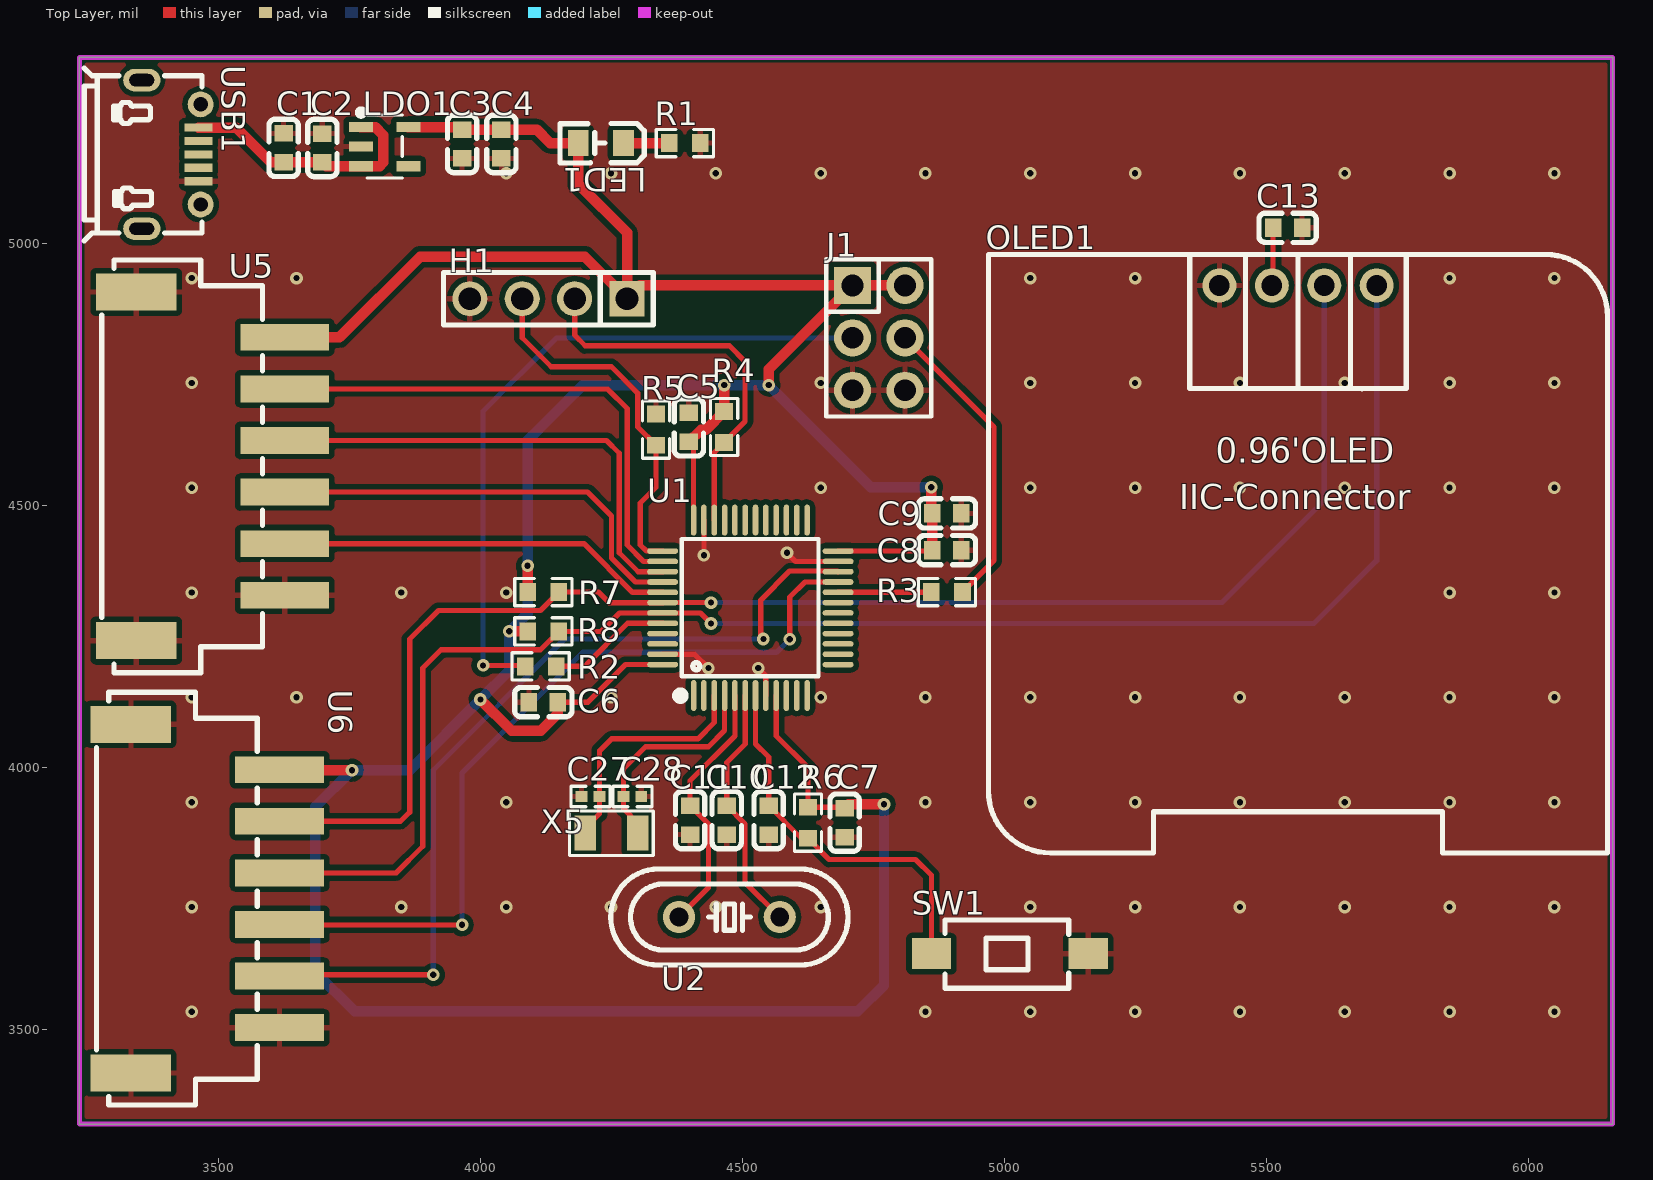
[diagram p0: Top Layer view]
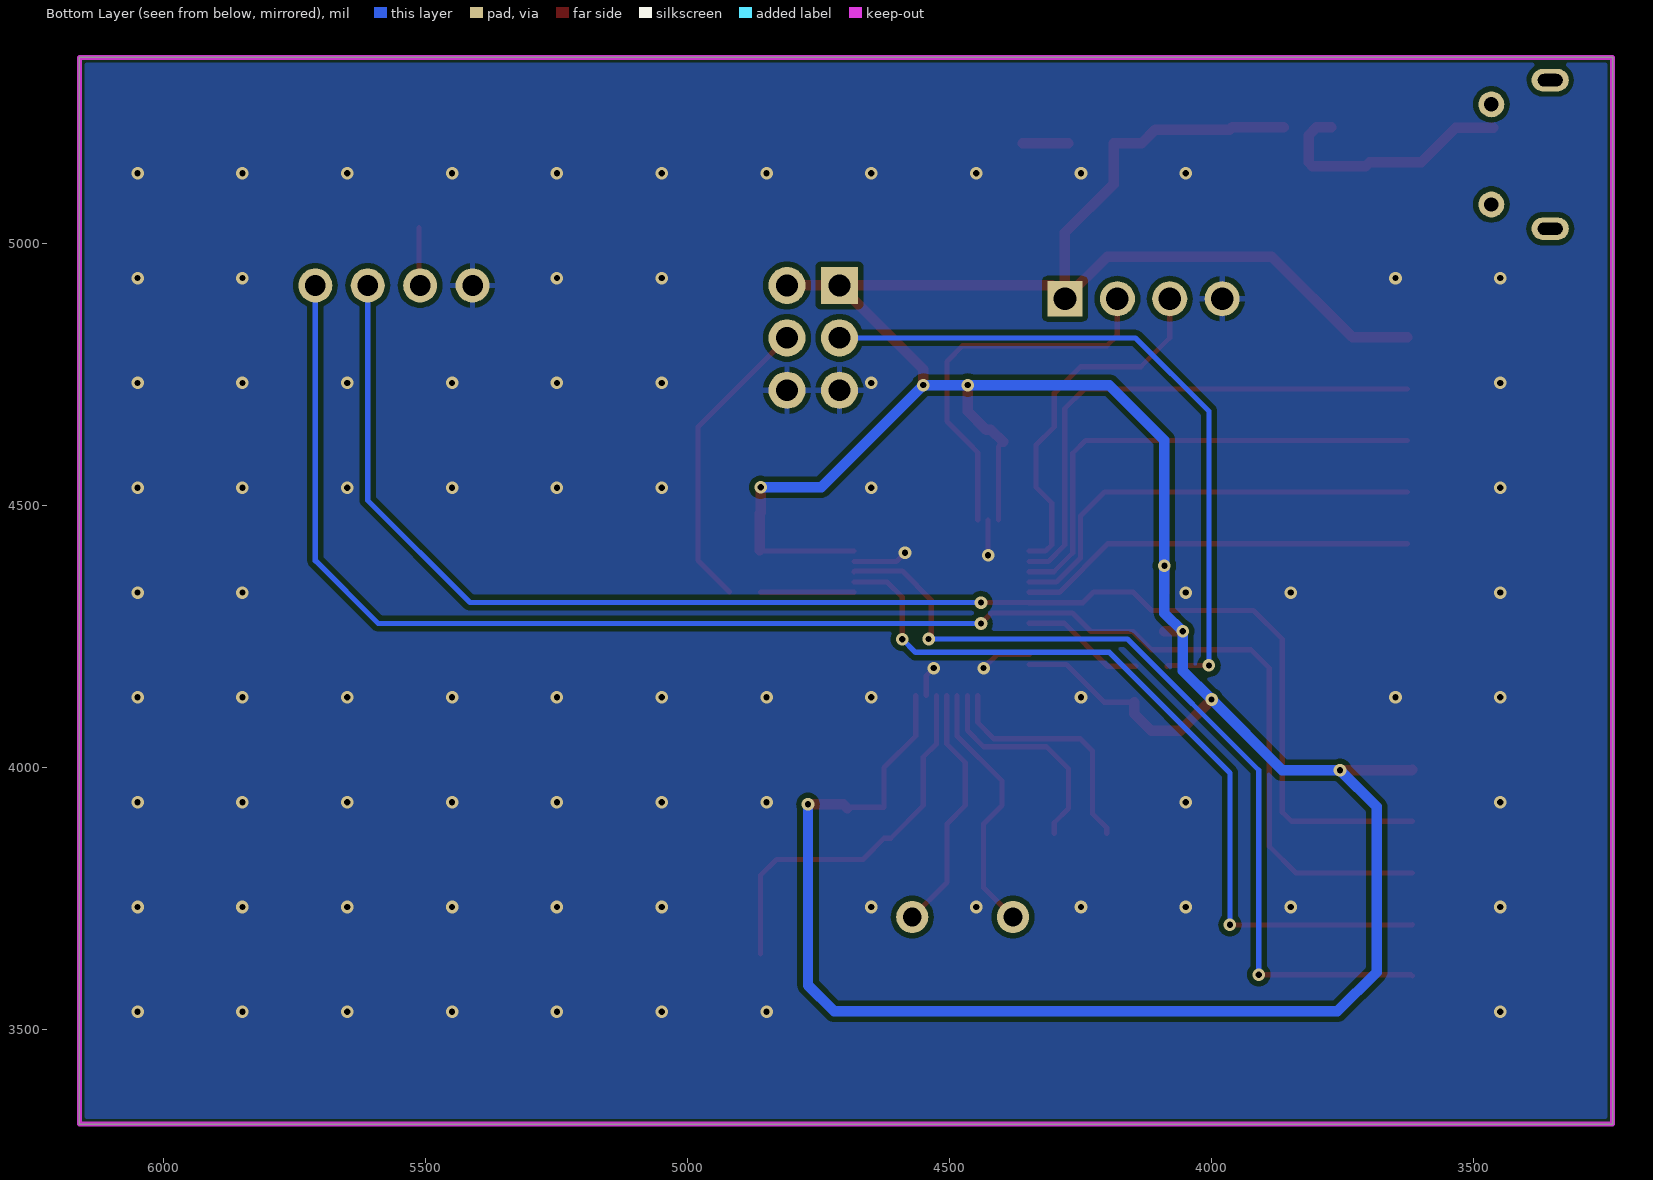
[diagram p1: Bottom Layer view, seen from below]
# Altium PCB MISC62287.pcbdoc
Units mil, origin at the board's own origin, x right, y up, seen from the top; angles counter-clockwise.
Board outline 2925 x 2035 mil, 2 copper layers (Top Layer, Bottom Layer), stack 62.206 mil thick; 35 components, 49 nets, 146 pads, 97 vias.

## Layer stack, top to bottom
Top Solder Mask Layer: solder mask 0.394, Dk 3.3
Top Layer: signal copper 1.379
Dielectric1: surface 59.449, FR4, Dk 4.5
Bottom Layer: signal copper 1.378
Bottom Solder Mask Layer: solder mask 0.394, Dk 3.3

## Board outline
3235,5355 3235,3320 6160,3320 6160,5355

## Design rules (kind name [scope] priority, off if disabled: settings)
BoardOutlineClearance copperThickness2oz_1 [All] p2 off: genericclearance=7.99 ignorepadtopadclearanceinfootprint=FALSE except(0: Arc-SplitContinuation Track-SplitContinuation SMDPad-SplitContinuation THPad-SplitContinuation Via-SplitContinuation Fill-SplitContinuation Region-SplitContinuation Poly-SplitContinuation Text-SplitContinuation Hole-SplitContinuation; 5.98: Arc-CutoutEdge SMDPad-CutoutEdge THPad-CutoutEdge Via-CutoutEdge Fill-CutoutEdge Region-CutoutEdge Text-CutoutEdge; 6.93: Hole-OutlineEdge Hole-CutoutEdge; 10: Poly-OutlineEdge Poly-CutoutEdge; 11.81: Arc-OutlineEdge Track-OutlineEdge SMDPad-OutlineEdge THPad-OutlineEdge Via-OutlineEdge Fill-OutlineEdge Region-OutlineEdge Text-OutlineEdge Track-CutoutEdge)
BoardOutlineClearance copperThickness1oz_1 [All] p4: genericclearance=4.02 ignorepadtopadclearanceinfootprint=FALSE except(0: Arc-SplitContinuation Track-SplitContinuation SMDPad-SplitContinuation THPad-SplitContinuation Via-SplitContinuation Fill-SplitContinuation Region-SplitContinuation Poly-SplitContinuation Text-SplitContinuation Hole-SplitContinuation; 6: SMDPad-CutoutEdge THPad-CutoutEdge Via-CutoutEdge Fill-CutoutEdge Region-CutoutEdge Text-CutoutEdge; 6.93: Hole-OutlineEdge Hole-CutoutEdge; 10: Poly-OutlineEdge Poly-CutoutEdge; 11.8: Arc-OutlineEdge Track-OutlineEdge SMDPad-OutlineEdge THPad-OutlineEdge Via-OutlineEdge Fill-OutlineEdge Region-OutlineEdge Text-OutlineEdge; 11.81: Arc-CutoutEdge Track-CutoutEdge)
Clearance copperThickness2oz [All] p1 off: gap=7.99 ignorepadtopadclearanceinfootprint=FALSE except(5.98: SMDPad-Track SMDPad-SMDPad THPad-Track SMDPad-THPad THPad-THPad Track-Via SMDPad-Via THPad-Via Via-Via Fill-Track Region-Track Fill-SMDPad Region-SMDPad Fill-THPad Region-THPad Fill-Via Region-Via Fill-Fill Fill-Region Region-Region Arc-Track Arc-SMDPad Arc-THPad Arc-Via Fill-Arc Region-Arc Arc-Arc Text-Track SMDPad-Text Text-THPad Text-Via Fill-Text Region-Text Arc-Text Text-Text; 6.93: Hole-Track Hole-SMDPad Hole-THPad Hole-Via Fill-Hole Region-Hole Hole-Arc Hole-Text; 10: Poly-Track Poly-SMDPad Poly-THPad Poly-Via Poly-Fill Poly-Region Poly-Poly Poly-Arc Poly-Text Poly-Hole)
Clearance copperThickness1oz [All] p3: gap=4.02 ignorepadtopadclearanceinfootprint=FALSE except(5.98: SMDPad-Track SMDPad-SMDPad THPad-Track SMDPad-THPad THPad-THPad Track-Via SMDPad-Via THPad-Via Via-Via Fill-Track Region-Track Fill-SMDPad Region-SMDPad Fill-THPad Region-THPad Fill-Via Region-Via Fill-Fill Fill-Region Region-Region; 6: Arc-Track Arc-SMDPad Arc-THPad Arc-Via Fill-Arc Region-Arc Arc-Arc Text-Track SMDPad-Text Text-THPad Text-Via Fill-Text Region-Text Arc-Text Text-Text; 6.93: Hole-Track Hole-SMDPad Hole-THPad Hole-Via Fill-Hole Region-Hole Hole-Arc Hole-Text; 10: Poly-Track Poly-SMDPad Poly-THPad Poly-Via Poly-Fill Poly-Region Poly-Poly Poly-Arc Poly-Text Poly-Hole)
DiffPairsRouting differentialPair [All] p1: maxlimit=6 minlimit=6 mostfreqgap=6 toplayer_minwidth=5 toplayer_prefwidth=10 toplayer_maxwidth=100 toplayer_mingap=6 toplayer_prefgap=6 toplayer_maxgap=6 bottomlayer_minwidth=5 bottomlayer_prefwidth=10 bottomlayer_maxwidth=100 bottomlayer_mingap=6 bottomlayer_prefgap=6 bottomlayer_maxgap=6 maxuncoupledlength=10
HoleToHoleClearance otherClearance [All] p1: gap=11.81 allowstackedmicrovias=TRUE
Length netLength [All] p1: minlimit=0 maxlimit=0
MatchedLengths netLengthTolerance [All] p1: tolerance=1000
PasteMaskExpansion pasteMaskExpansion [All] p1: expansion=0
PlaneConnect innerPlane [All] p1: planeconnectstyle=Relief reliefexpansion=20 reliefentries=4 reliefconductorwidth=10 reliefairgap=10
PolygonConnect copperRegion [(InNet('GND'))] p1: connectstyle=Relief reliefconductorwidth=10 reliefentries=4 polygonreliefangle="90 Angle" airgapwidth=10 via.connectstyle=Relief via.reliefconductorwidth=10 via.reliefentries=4 via.polygonreliefangle="90 Angle" via.airgapwidth=10
RoutingVias viaSize [All] p1: holewidth=12.01 width=24.02 viastyle="Through Hole" minholewidth=11.81 minwidth=19.68 maxholewidth=248.03 maxwidth=393.7
SolderMaskExpansion solderMaskExpansion [IsVia] p1: expansion=-1000 istentingtop=TRUE
SolderMaskExpansion solderMaskExpansion [All] p2: expansion=2 istentingtop=FALSE
Width copperThickness2oz_2 [All] p1 off: maxlimit=100 minlimit=8 preferedwidth=10
Width copperThickness1oz_2 [All] p2: maxlimit=100 minlimit=5 preferedwidth=10

## Components (designator, comment, footprint, x,y, rotation, side; value= is the part's Value field where it differs from the comment)
C1 "0.1UF" C0603 3624.41,5182.46 r270 top
C2 "1uF" C0603 3698.42,5182.34 r270 top
C3 "0.1UF" C0603 3965,5190 r90 top
C4 "1uF" C0603 4040,5190 r90 top
C5 "100nF" C0603 4397.65,4649.18 r270 top
C6 "100nF" C0603 4120,4125 r0 top
C7 "100nF" C0603 4695,3895 r90 top
C8 "100nF" C0603 4890,4415 r180 top
C9 "100nF" C0603 4890,4485 r180 top
C10 "1uF" C0603 4470,3900 r270 top
C11 "1uF" C0603 4400,3900 r270 top
C12 "0.1UF" C0603 4550,3900 r90 top
C13 "0.1UF" C0603 5540,5030 r0 top
C27 "12pF" R0402 4210,3945 r0 top
C28 "12pF" R0402 4290,3945 r180 top
H1 "PZ254V-11-04P" HDR-TH_4P-P2.54-V-M 4129.75,4894.66 r180 top
J1 "2.54-2*3P pin header" HDR-TH_6P-P2.54-V-M-R2-C3-S2.54-1 4760,4820 r270 top
LDO1 "ME6211C33M5G-N" SOT-23-5_L3.0-W1.7-P0.95-LS2.8-BL 3817.21,5184.9 r270 top
LED1 "NCD0805R1" LED0805-RD 4229.75,5191.65 r180 top
OLED1 "0.96OLED_4P_MODULE_JX" 0.96OLED_4P 5560,4920 r0 top
R1 "1K" R0603 4389.91,5191.65 r0 top
R2 "10kΩ" R0603 4114.93,4193.27 r180 top
R3 "10kΩ" R0603 4890,4335 r180 top
R4 "10K" R0603 4465,4650 r90 top
R5 "10K" R0603 4335,4645 r270 top
R6 "10K" R0603 4625,3895 r90 top
R7 "4.7K" R0603 4120,4335 r180 top
R8 "4.7K" R0603 4120,4260 r180 top
SW1 "KEY_RESET" SW-SMD_L6.0-W3.3-LS8.0 5010,3645 r0 top
U1 "STM32F103C8T6" LQFP-48_L7.0-W7.0-P0.50-LS9.0-BL 4515,4305 r0 top
U2 "8M crystal" HC-49S_L11.5-W4.7-P4.88 4475,3715 r0 top
U5 "XH2.54mm-LI-6P" CONN-SMD_6P-P2.50-H 3485,4575 r270 top
U6 "XH2.54mm-LI-6P" CONN-SMD_6P-P2.50-H 3475,3750 r270 top
USB1 "MICRO-USB-1" MICRO-USB-SMD_C9900008946 3410,5170 r270 top
X5 "32.768kHz" OSC-SMD_L3.2-W1.5 4250,3875 r0 top

## Footprints (in the part's own frame and the unit in brackets; to place one, negate y for a bottom-side part, rotate by r counter-clockwise, add the part's x,y. Pads: shape width x height; smd on the part's side, far side on the other; paste and mask are expansions set on the pad)
0.96OLED_4P [mm]
  round 1.65 hole 1 copper offset 0,0: 1(-3.81,-0.001) 2(-1.27,0.002) 3(1.27,0.002) 4(3.81,0.002)
  silkscreen extent -15,-27.5 15,1.5
C0603 [mm]
  rect 0.8x0.9 smd: 1(-0.7,0) 2(0.7,0)
  silkscreen extent -1.39,-0.71 1.39,0.71
CONN-SMD_6P-P2.50-H [mm]
  rect 1.3x4.3 smd paste+0 mask+0.05: 1(-6.25,3.6) 2(-3.75,3.6) 3(-1.25,3.6) 4(1.25,3.6) 5(3.75,3.6) 6(6.25,3.6)
  rect 1.8x3.9 smd paste+0 mask+0.05: 7(-8.45,-3.6) 8(8.45,-3.6)
  silkscreen extent -10,-5.27 10,2.52
HC-49S_L11.5-W4.7-P4.88 [mm]
  round 1.56 hole 0.9: 1(-2.44,0) 2(2.44,0)
  silkscreen extent -5.75,-2.33 5.75,2.33
HDR-TH_4P-P2.54-V-M [mm]
  rect 1.7x1.7 hole 1.1: 1(-3.81,0)
  round 1.7 hole 1.1: 2(-1.27,0) 3(1.27,0) 4(3.81,0)
  silkscreen extent -5.08,-1.27 5.08,1.27
HDR-TH_6P-P2.54-V-M-R2-C3-S2.54-1 [mm]
  rect 1.8x1.8 hole 1.05: 1(-2.54,-1.27)
  round 1.8 hole 1.05: 2(-2.54,1.27) 3(0,-1.27) 4(0,1.27) 5(2.54,-1.27) 6(2.54,1.27)
  silkscreen extent -3.81,-2.54 3.81,2.54
LED0805-RD [mm]
  rect 1x1.25 smd: 1(-1.1,0) 2(1.1,0)
  silkscreen extent -2.1,-0.95 1.98,0.96
LQFP-48_L7.0-W7.0-P0.50-LS9.0-BL [mm]
  oval 0.27x1.5 smd paste+0 mask+0.05: 1(-2.75,-4.25) 2(-2.25,-4.25) 3(-1.75,-4.25) 4(-1.25,-4.25) 5(-0.75,-4.25) 6(-0.25,-4.25) 7(0.25,-4.25) 8(0.75,-4.25) 9(1.25,-4.25) 10(1.75,-4.25) 11(2.25,-4.25) 12(2.75,-4.25) 25(2.75,4.25) 26(2.25,4.25) 27(1.75,4.25) 28(1.25,4.25) 29(0.75,4.25) 30(0.25,4.25) 31(-0.25,4.25) 32(-0.75,4.25) 33(-1.25,4.25) 34(-1.75,4.25) 35(-2.25,4.25) 36(-2.75,4.25)
  oval 1.5x0.27 smd paste+0 mask+0.05: 13(4.25,-2.75) 14(4.25,-2.25) 15(4.25,-1.75) 16(4.25,-1.25) 17(4.25,-0.75) 18(4.25,-0.25) 19(4.25,0.25) 20(4.25,0.75) 21(4.25,1.25) 22(4.25,1.75) 23(4.25,2.25) 24(4.25,2.75) 37(-4.25,2.75) 38(-4.25,2.25) 39(-4.25,1.75) 40(-4.25,1.25) 41(-4.25,0.75) 42(-4.25,0.25) 43(-4.25,-0.25) 44(-4.25,-0.75) 45(-4.25,-1.25) 46(-4.25,-1.75) 47(-4.25,-2.25) 48(-4.25,-2.75)
  silkscreen extent -3.59,-4.46 3.3,3.34
MICRO-USB-SMD_C9900008946 [mm]
  rect 0.4x1.35 smd paste-100 mask+0.051: 1(-1.3,1.325) 2(-0.65,1.325) 3(0,1.325) 4(0.65,1.325) 5(1.3,1.325)
  oval 1.1x1.8 hole 0.6 slot 1.2 at 90 deg: 6(-3.6,-1.425) 6(3.6,-1.425)
  round 1.25 hole 0.7: 6(-2.425,1.425) 6(2.425,1.425)
  silkscreen extent -4.19,-4.22 4.19,1.5
OSC-SMD_L3.2-W1.5 [mm]
  rect 1.05x1.7 smd: 1(-1.275,0) 2(1.275,0)
  silkscreen extent -2.03,-1.08 2.03,1.08
R0402 [mm]
  rect 0.566x0.54 smd paste-100 mask+0.051: 1(-0.433,0) 2(0.433,0)
  silkscreen extent -0.94,-0.5 0.94,0.5
R0603 [mil]
  rect 31.75x34.02 smd paste-3937.01 mask+2: 1(-29.66,0) 2(29.66,0)
  silkscreen extent -55,-26 55,26
SOT-23-5_L3.0-W1.7-P0.95-LS2.8-BL [mm]
  rect 0.49x1.157 smd: 1(-0.95,-1.154) 2(0,-1.154) 3(0.95,-1.154)
  rect 0.49x1.175 smd: 4(0.95,1.154) 5(-0.95,1.154)
  silkscreen extent -1.8,-1.29 1.53,0.85
SW-SMD_L6.0-W3.3-LS8.0 [mm]
  rect 1.9x1.5 smd: 1(-3.8,0) 2(3.8,0)
  silkscreen extent -3.14,-1.67 2.86,1.63

## Via types
v1: diameter 24.02, hole 12, Top Layer to Bottom Layer, 97 vias

## Nets (pads, with @x,y where several pads share a name; then routed paths per layer and width w, separated by ;. In a path a pad name is that pad's centre, name@x,y a point inside that pad or via, vN(x,y) a via of type N, cw(c..) or ccw(c..) an arc to the next point about the centre after c; other vN are vias at no path point)
$1N10: LED1.1 R1.1 | length 87.2
  Top Layer w20: LED1.1 R1.1
$1N21: J1.3 R2.2 | length 1329
  Top Layer w10: v1(4005,4195) 4083.53,4195 R2.2
  Bottom Layer w10: v1(4005,4195) 4005,4680 4145,4820 J1.3
$1N22: J1.4 R3.1 | length 580.4
  Top Layer w10: J1.4 4980,4650 4980,4395.34 R3.1
+5V: C1.2 C2.2 LDO1.1 LDO1.3 USB1.1 | length 512
  Top Layer w20: USB1.1 3533.82,5221.18 3600.1,5154.9 ; C1.2 3600.1,5154.9 ; LDO1.1 3799.18,5222.3 3815,5206.48 3815,5155 3807.5,5147.5 LDO1.3 3705.7,5147.5 C2.2 3600.22,5154.78 3600.1,5154.9
BOOT0: R2.1 U1.44 | length 237.1
  Top Layer w10: R2.1 4198.27,4193.27 4280.47,4275.47 U1.44
BOOT1: R3.2 U1.20 | length 178.2
  Top Layer w10: U1.20 4859.87,4334.53 R3.2
D+: USB1.3
D-: USB1.2
GND: C1.1 C2.1 C3.1 C4.1 C5.1 C6.1 C7.1 C8.1 C9.1 C10.2 C11.2 C12.1 C13.2 C27.1 C28.1 H1.4 J1.5 J1.6 LDO1.2 OLED1.1 R1.2 R5.1 SW1.2 U1.8 U1.23 U1.35 U1.47 U5.6 U5.7 U5.8 U6.6 U6.7 U6.8 USB1.5 | length 328
  Top Layer w10: U1.47 4408.58,4216.42 v1(4435,4190) ; v1(4426.42,4405) U1.35 ; v1(4530,4190) 4544.53,4175.47 U1.8 ; v1(4585,4410) 4601.42,4393.58 U1.23
  other v1: 3449.1,3534.1 4849.1,3534.1 5049.1,3534.1 5249.1,3534.1 5449.1,3534.1 5649.1,3534.1 5849.1,3534.1 6049.1,3534.1 3449.1,3734.1 3849.1,3734.1 4049.1,3734.1 4249.1,3734.1 4449.1,3734.1 4649.1,3734.1 5049.1,3734.1 5249.1,3734.1 5449.1,3734.1 5649.1,3734.1 5849.1,3734.1 6049.1,3734.1 3449.1,3934.1 4049.1,3934.1 4849.1,3934.1 5049.1,3934.1 5249.1,3934.1 5449.1,3934.1 5649.1,3934.1 5849.1,3934.1 6049.1,3934.1 3449.1,4134.1 3649.1,4134.1 4249.1,4134.1 4649.1,4134.1 4849.1,4134.1 5049.1,4134.1 5249.1,4134.1 5449.1,4134.1 5649.1,4134.1 5849.1,4134.1 6049.1,4134.1 3449.1,4334.1 3849.1,4334.1 4049.1,4334.1 5849.1,4334.1 6049.1,4334.1 3449.1,4534.1 4649.1,4534.1 5049.1,4534.1 5249.1,4534.1 5449.1,4534.1 5649.1,4534.1 5849.1,4534.1 6049.1,4534.1 3449.1,4734.1 4649.1,4734.1 5049.1,4734.1 5249.1,4734.1 5449.1,4734.1 5649.1,4734.1 5849.1,4734.1 6049.1,4734.1 3449.1,4934.1 3649.1,4934.1 5049.1,4934.1 5249.1,4934.1 5849.1,4934.1 6049.1,4934.1 4049.1,5134.1 4249.1,5134.1 4449.1,5134.1 4649.1,5134.1 4849.1,5134.1 5049.1,5134.1 5249.1,5134.1 5449.1,5134.1 5649.1,5134.1 5849.1,5134.1 6049.1,5134.1
OSC32_IN: C27.2 U1.3 X5.1 | length 461.4
  Top Layer w10: X5.1 4199.8,3884.8 4227.04,3912.04 C27.2 4227.04,4032.04 4250,4055 4415,4055 4446.1,4086.1 U1.3
OSC32_OUT: C28.2 U1.4 X5.2 | length 424.1
  Top Layer w10: X5.2 4300.2,3894.8 4272.96,3922.04 C28.2 4272.96,3997.96 4315,4040 4435,4040 4465.79,4070.79 U1.4
OSCIN: C11.1 U1.5 U2.1 | length 495.8
  Top Layer w10: U2.1 4435,3771.06 4435,3892.56 C11.1 4400,3975 4485.47,4060.47 U1.5
OSOUT: C10.1 U1.6 U2.2 | length 479.1
  Top Layer w10: U1.6 4505.16,4045.16 4470,4010 C10.1 4505,3892.56 4505,3781.06 U2.2
PA0: U1.10
PA1: U1.11
PA2: U1.12
PA3: U1.13
PA4: U1.14
PA5: U1.15
PA6: U1.16
PA7: U1.17
PA8: U1.29
PA9: U1.30
PA10: U1.31
PA11: U1.32
PA12: U1.33
PA15: U1.38 U5.2 | length 1009.6
  Top Layer w10: U5.2 4242.35,4722.65 4280,4685 4280,4425 4311.42,4393.58 U1.38
PB0: U1.18
PB1: U1.19
PB3: U1.39 U5.3 | length 935.9
  Top Layer w10: U5.3 4240.78,4624.22 4265,4600 4265,4410 4301.1,4373.9 U1.39
PB4: U1.40 U5.4 | length 838.9
  Top Layer w10: U5.4 4204.2,4525.8 4250,4480 4250,4400 4295.79,4354.21 U1.40
PB5: U1.41 U5.5 | length 759.4
  Top Layer w10: U5.5 4197.63,4427.37 4290.47,4334.53 U1.41
PB6: OLED1.3 R7.1 U1.42 U6.2 | length 2867
  Top Layer w10: U6.2 3847.65,3897.65 3865,3915 3865,4245 3920,4300 4114.66,4300 R7.1 4225,4335 4245.16,4314.84 U1.42 4347.84,4315 v1(4440,4315)
  Bottom Layer w10: v1(4440,4315) 5415,4315 5610,4510 OLED1.3@5610,4920.05
PB7: OLED1.4 R8.1 U1.43 U6.3 | length 3081
  Top Layer w10: U6.3 3839.22,3799.22 3890,3850 3890,4190 3925,4225 4114.66,4225 R8.1 4230,4260 4265.16,4295.16 U1.43 4419.84,4295.16 v1(4440,4275)
  Bottom Layer w10: v1(4440,4275) 5590,4275 5710,4395 OLED1.4@5710,4920.05
PB8: U1.45
PB9: U1.46
PB10: U1.21 U6.4 | length 1553.6
  Top Layer w10: U6.4 3617.54,3700 v1(3965,3700) ; v1(4590,4245) 4590,4325 4619.21,4354.21 U1.21
  Bottom Layer w10: v1(3965,3700) 3965,3990 4195,4220 4565,4220 v1(4590,4245)
PB11: U1.22 U6.5 | length 1668.9
  Top Layer w10: U6.5 3619.37,3605 v1(3910,3605) ; v1(4540,4245.55) 4539.45,4245 4535,4245 4535,4320 4590,4375 4681.22,4375 U1.22
  Bottom Layer w10: v1(3910,3605) 3910,3995 4160.55,4245.55 v1(4540,4245.55)
PB12: U1.25
PB13: U1.26
PB14: U1.27
PB15: U1.28
PC13: U1.2
RESET: C12.2 R6.1 SW1.1 U1.7 | length 735.6
  Top Layer w10: U1.7 4524.84,4045.16 4550,4020 C12.2 4612.22,3865.34 R6.1 4665.34,3825 4830,3825 4860.39,3794.61 SW1.1
SWCLK: H1.3 R5.2 U1.37 | length 702.7
  Top Layer w10: H1.3 4079.75,4820.25 4135,4765 4250,4765 4300,4715 4300,4650.34 R5.2 4335,4535 4305,4505 4305,4425 4316.73,4413.27 U1.37
SWIO: H1.2 R4.1 U1.34 | length 742.6
  Top Layer w10: H1.2 4179.75,4825.25 4200,4805 4475,4805 4505,4775 4505,4660.34 R4.1 4446.1,4601.44 U1.34
VBAT: U1.1
VCC: C3.2 C4.2 C5.2 C6.2 C7.2 C8.2 C9.2 H1.1 J1.1 J1.2 LDO1.5 LED1.2 R4.2 R6.2 R7.2 R8.2 U1.9 U1.24 U1.36 U1.48 U5.1 U6.1 | length 7488.6
  Top Layer w10: C6.2 4205,4125 4276.73,4196.73 U1.48 ; C5.2 4406.73,4612.54 U1.36 ; U1.9 4564.21,4060.79 4625,4000 R6.2 4692.9,3924.66 C7.2 ; U1.24 4860.71,4413.27 C8.2
  Top Layer w20: U6.1 3617.81,3995 v1(3755,3995) ; U5.1 3731.07,4821.07 3885,4975 4199.4,4975 H1.1 ; LDO1.5 3960.26,5222.3 C3.2 C4.2 4107.44,5217.56 4133.36,5191.64 LED1.2 4186.44,5113.56 4279.75,5020.25 H1.1 ; v1(4000,4130) 4060,4070 4115,4070 4147.56,4102.56 C6.2 ; v1(4055,4260) R8.2 ; v1(4090,4385) 4090,4335.34 R7.2 ; C5.2 4421.03,4645 4430.34,4645 R4.2 v1(4465,4730) ; v1(4550,4730) 4550,4760 J1.1 ; C7.2 4702.44,3930 v1(4770,3930) ; J1.2 J1.1 ; v1(4860,4535) 4860,4487.44 C9.2 C8.2 ; H1.1 4305.09,4920 J1.1
  Bottom Layer w20: v1(4770,3930) 4770,3585 4720,3535 3760,3535 3685,3610 3685,3925 v1(3755,3995) 3865,3995 v1(4000,4130) 4055,4185 v1(4055,4260) 4090,4295 v1(4090,4385) 4090,4625 4195,4730 v1(4465,4730) v1(4550,4730) 4745,4535 v1(4860,4535)
VCC+3.3V: C13.1 OLED1.2 | length 111
  Top Layer w10: OLED1.2@5510,4920.05 5512.44,4922.49 C13.1
pads on no net: LDO1.4 USB1.4 USB1.6

## Polygon pours and split planes (outlines as drawn)
GND on Top Layer (solid, remove dead copper, pour order 0): 3000,5585 3000,3000 6480,3000 6480,5585
GND on Bottom Layer (solid, remove dead copper, pour order 2): 3060,5520 3060,3250 6440,3250 6440,5520

## Keep-outs
Board Outline Layer:
  the board outline again, w10